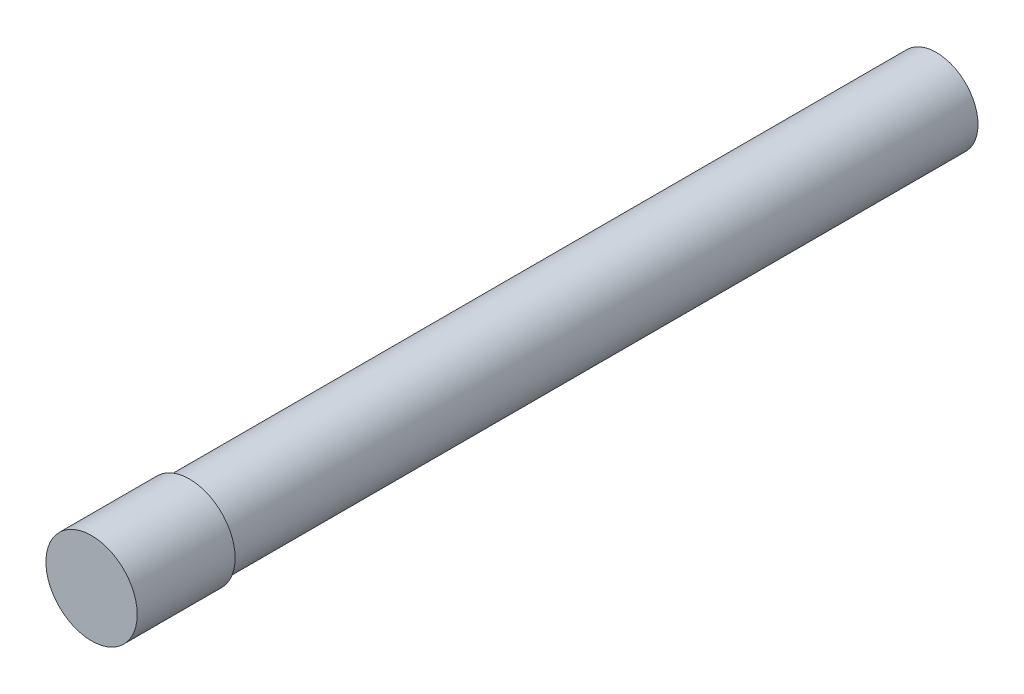
SolidWorks part; units mm, degrees
ref_plane "Front Plane" through (0, 0, 0) normal (0, 0, 1) x (1, 0, 0)
ref_plane "Top Plane" through (0, 0, 0) normal (0, 1, 0) x (1, 0, 0)
ref_plane "Right Plane" through (0, 0, 0) normal (1, 0, 0) x (0, 0, -1)
other "Configuration Table"
sketch "Sketch1" plane through (0, 0, 0) normal (0, 0, 1) x (1, 0, 0)
  circle A0 centre (0, 0) radius 25.082
extrude "Boss-Extrude1" add sketch "Sketch1" against normal blind 450
sketch "Sketch2" plane through (0, 0, 0) normal (0, 0, 1) x (1, 0, 0)
  circle A0 centre (0, 0) radius 27.5
  dimension "D1" = 55
extrude "Boss-Extrude2" add sketch "Sketch2" along normal up to surface (59 mm away)
